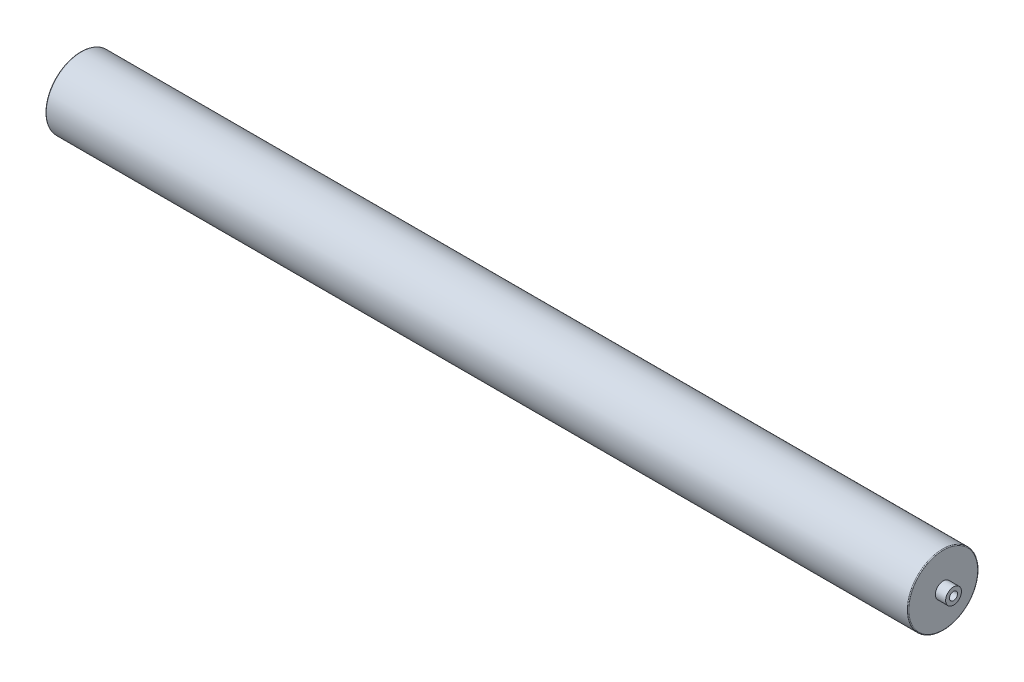
from build123d import *

# Parameters (mm, degrees)
SKETCH1_R                        = 44.5
BOSS_EXTRUDE1_DEPTH              = 545
SKETCH2_R                        = 10
BOSS_EXTRUDE2_DEPTH              = 13
BOSS_EXTRUDE3_START              = 13
SKETCH3_R                        = 10
BOSS_EXTRUDE3_DEPTH              = 13
FILLET1_R                        = 1
M12_TAPPED_HOLE1_D               = 10.2
M12_TAPPED_HOLE1_DEPTH           = 20
M12_TAPPED_HOLE1_TIP             = 3.064389157
M12_TAPPED_HOLE1_ON_FACE_2_D     = 10.2
M12_TAPPED_HOLE1_ON_FACE_2_DEPTH = 20
M12_TAPPED_HOLE1_ON_FACE_2_TIP   = 3.064389157


with BuildPart() as part:
    # Sketch1 → Boss-Extrude1 (new, symmetric)
    with BuildSketch(Plane(origin=(0, 0, 0), x_dir=(0, 0, -1), z_dir=(1, 0, 0))):
        Circle(SKETCH1_R)
    extrude(amount=BOSS_EXTRUDE1_DEPTH, both=True)

    # Sketch2 → Boss-Extrude2 (add)
    with BuildSketch(Plane(origin=(545, 0, 0), x_dir=(0, 0, -1), z_dir=(1, 0, 0))):
        with Locations(Location((0, 0, 0), (0, 0, 180))):
            Circle(SKETCH2_R)
    extrude(amount=BOSS_EXTRUDE2_DEPTH)

    # Sketch3 → Boss-Extrude3 (add)
    with BuildSketch(Plane.ZY.offset(545).offset(BOSS_EXTRUDE3_START)):
        Circle(SKETCH3_R)
    extrude(amount=-BOSS_EXTRUDE3_DEPTH)

    # Fillet1
    fillet1_edges = [part.edges().sort_by_distance(p)[0] for p in [
        (-545, 0, 44.5),
        (545, 0, 44.5),
    ]]
    fillet(fillet1_edges, radius=FILLET1_R)

    # M12 Tapped Hole1
    with Locations(Plane(origin=(558, 0, 0), x_dir=(0, 0, 1), z_dir=(1, 0, 0))):
        with Locations((0, 0)):
            Hole(M12_TAPPED_HOLE1_D / 2, depth=M12_TAPPED_HOLE1_DEPTH)
            with Locations((0, 0, -(M12_TAPPED_HOLE1_DEPTH + M12_TAPPED_HOLE1_TIP / 2))):  # 118° drill point
                Cone(0, M12_TAPPED_HOLE1_D / 2, M12_TAPPED_HOLE1_TIP, mode=Mode.SUBTRACT)

    # M12 Tapped Hole1 on face 2
    with Locations(Plane(origin=(-558, 0, 0), x_dir=(0, 0, -1), z_dir=(-1, 0, 0))):
        with Locations((0, 0)):
            Hole(M12_TAPPED_HOLE1_ON_FACE_2_D / 2, depth=M12_TAPPED_HOLE1_ON_FACE_2_DEPTH)
            with Locations((0, 0, -(M12_TAPPED_HOLE1_ON_FACE_2_DEPTH + M12_TAPPED_HOLE1_ON_FACE_2_TIP / 2))):  # 118° drill point
                Cone(0, M12_TAPPED_HOLE1_ON_FACE_2_D / 2, M12_TAPPED_HOLE1_ON_FACE_2_TIP, mode=Mode.SUBTRACT)


solid = part.part
